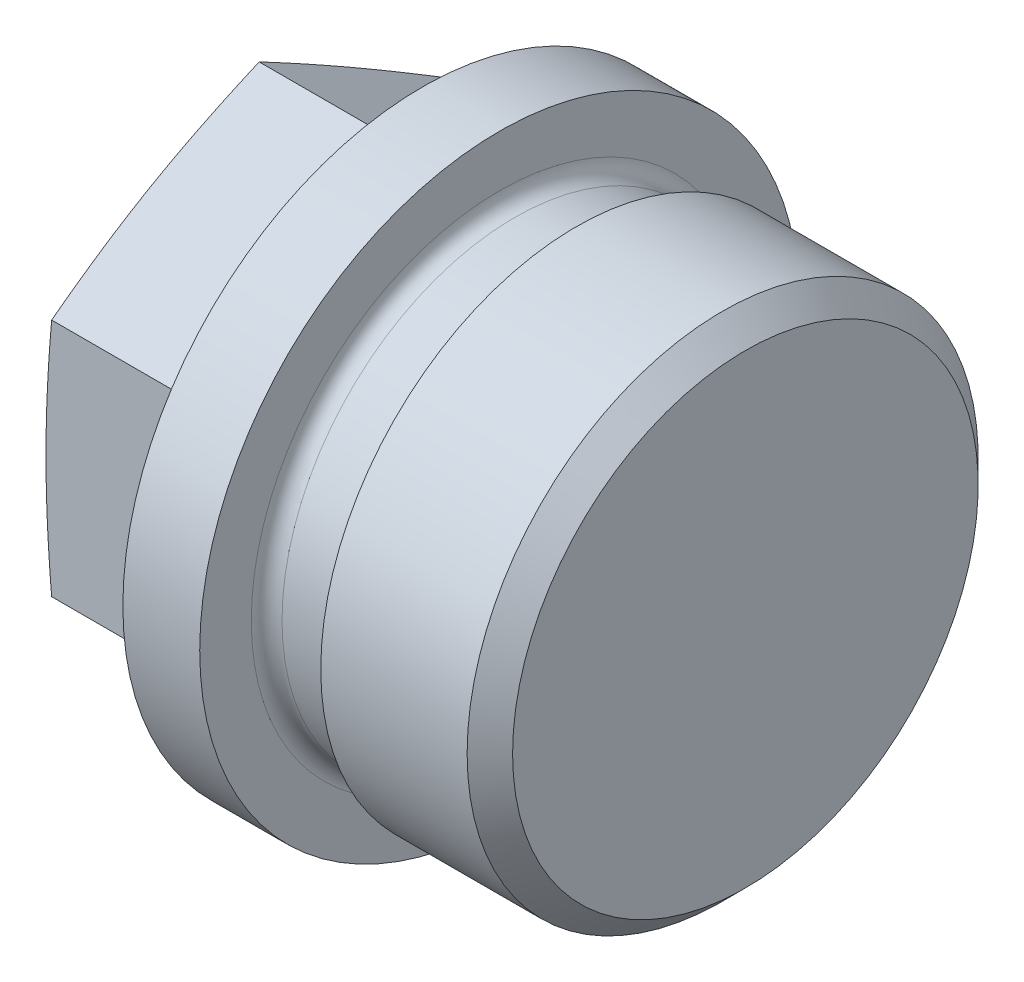
SolidWorks part; units mm, degrees
material "35钢"
ref_plane "Front Plane" through (0, 0, 0) normal (0, 0, 1) x (1, 0, 0)
ref_plane "Top Plane" through (0, 0, 0) normal (0, 1, 0) x (1, 0, 0)
ref_plane "Right Plane" through (0, 0, 0) normal (1, 0, 0) x (0, 0, -1)
sketch "Sketch1" plane through (0, 0, 0) normal (0, 0, 1) x (1, 0, 0)
  line L0 (0, 0) -> (32, 0) construction
  line L1 (32, 0) -> (32, 16.6245) construction
  line L2 (32, 16.6245) -> (21, 16.6245) construction
  line L3 (21, 16.6245) -> (21, 15.1455)
  line L4 (21, 15.1455) -> (16, 15.1455)
  line L5 (16, 15.1455) -> (16, 19.5)
  line L6 (16, 19.5) -> (11, 19.5)
  line L7 (11, 19.5) -> (11, 1.5)
  line L8 (11, 1.5) -> (0, 1.5)
  line L9 (0, 1.5) -> (0, 0)
  line L10 (0, 0) -> (32, 0)
  line L11 (30.521, 16.6245) -> (32, 15.1455)
  line L12 (21, 16.6245) -> (30.521, 16.6245)
  line L13 (32, 15.1455) -> (32, 0)
  dimension "L" = 32
  dimension "b" = 5
  dimension "1" = 16
  dimension "d" = 33.249
  dimension "Do" = 39
  dimension "D6" = 3
  dimension "d1" = 30.291
  dimension "D8" = 45
revolve "Revolve1" add sketch "Sketch1" angle 360 about L0
sketch "Sketch2" plane through (0, 0, 0) normal (-1, 0, 0) x (0, 0, 1)
  line L1 (0, 15.5885) -> (-13.5, 7.7942)
  line L2 (-13.5, 7.7942) -> (-13.5, -7.7942)
  line L3 (-13.5, -7.7942) -> (0, -15.5885)
  line L4 (0, -15.5885) -> (13.5, -7.7942)
  line L5 (13.5, -7.7942) -> (13.5, 7.7942)
  line L6 (13.5, 7.7942) -> (0, 15.5885)
  circle A0 centre (0, 0) radius 13.5 construction
  dimension "s" = 27
extrude "Extrude1" add sketch "Sketch2" against normal up to surface (11 mm away) up to face at (11, 0, 1.5)
sketch "Sketch3" plane through (0, 0, 0) normal (-1, 0, 0) x (0, 0, 1)
  circle A0 centre (0, 0) radius 13.5 construction
  circle A1 centre (0, 0) radius 13.5
extrude "Cut-Extrude1" cut sketch "Sketch3" against normal blind 10 draft 80 flip side to cut
fillet "Fillet1" radius 1 2 edges at (21, 0, 15.1455) (16, 0, 15.1455)
